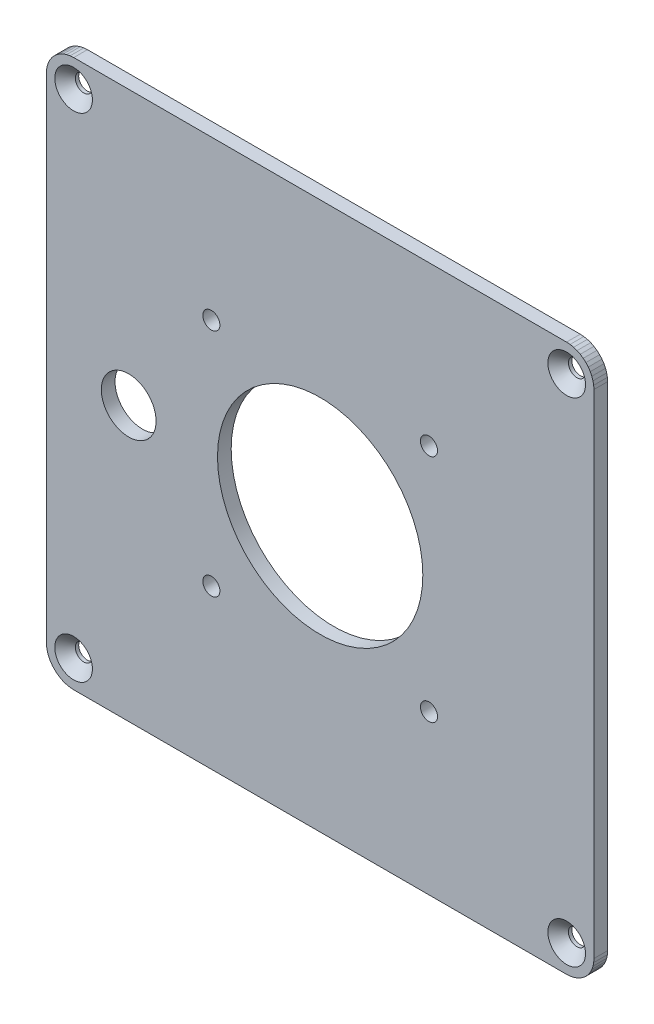
from build123d import *

# Parameters (mm, degrees)
BOSS_EXTRUDE1_DEPTH     = 2
CUT_EXTRUDE1_DEPTH      = 57.603885529
CUT_EXTRUDE1_DEPTH_BACK = 57.603885529
SKETCH2_R               = 15
SKETCH3_R               = 4
CUT_EXTRUDE2_DEPTH      = 10
SKETCH4_R               = 1.25
CUT_EXTRUDE3_DEPTH      = 10
SKETCH5_R               = 2
CUT_EXTRUDE4_DEPTH      = 10
MOVE_FACE1_BY           = 0.75
MOVE_FACE1_2_BY         = 0.75
MOVE_FACE1_3_BY         = 0.75
MOVE_FACE1_4_BY         = 0.75
CHAMFER1_SIZE           = 1.5


with BuildPart() as part:
    # Sketch1 → Boss-Extrude1 (new body)
    with BuildSketch(Plane.XY.offset(196.776792407)):
        Polygon((-39.999999106, -35.99999845), (-39.965778589, -36.522105336), (-39.863705635, -37.035275251), (-39.695519954, -37.530735135), (-39.464101195, -37.999998778), (-39.173413068, -38.43504563), (-38.828425109, -38.828425109), (-38.43504563, -39.173413068), (-37.999998778, -39.464101195), (-37.530735135, -39.695519954), (-37.035275251, -39.863705635), (-36.522105336, -39.965778589), (-35.99999845, -39.999999106), (35.99999845, -39.999999106), (36.522105336, -39.965778589), (37.035275251, -39.863705635), (37.530735135, -39.695519954), (37.999998778, -39.464101195), (38.43504563, -39.173413068), (38.828425109, -38.828425109), (39.173413068, -38.43504563), (39.464101195, -37.999998778), (39.695519954, -37.530735135), (39.863705635, -37.035275251), (39.965778589, -36.522105336), (39.999999106, -35.99999845), (39.999999106, 35.99999845), (39.965778589, 36.522105336), (39.863705635, 37.035275251), (39.695519954, 37.530735135), (39.464101195, 37.999998778), (39.173413068, 38.43504563), (38.828425109, 38.828425109), (38.43504563, 39.173413068), (37.999998778, 39.464101195), (37.530735135, 39.695519954), (37.035275251, 39.863705635), (36.522105336, 39.965778589), (35.99999845, 39.999999106), (-35.99999845, 39.999999106), (-36.522105336, 39.965778589), (-37.035275251, 39.863705635), (-37.530735135, 39.695519954), (-37.999998778, 39.464101195), (-38.43504563, 39.173413068), (-38.828425109, 38.828425109), (-39.173413068, 38.43504563), (-39.464101195, 37.999998778), (-39.695519954, 37.530735135), (-39.863705635, 37.035275251), (-39.965778589, 36.522105336), (-39.999999106, 35.99999845), align=None)
        Polygon((-37.448886782, -36.388229579), (-37.50000149, -35.99999845), (-37.448886782, -35.611771047), (-37.29903698, -35.250000656), (-37.060663104, -34.939337522), (-36.74999997, -34.700963646), (-36.388229579, -34.551113844), (-35.99999845, -34.499999136), (-35.611771047, -34.551113844), (-35.250000656, -34.700963646), (-34.939337522, -34.939337522), (-34.700963646, -35.250000656), (-34.551113844, -35.611771047), (-34.499999136, -35.99999845), (-34.551113844, -36.388229579), (-34.700963646, -36.74999997), (-34.939337522, -37.060663104), (-35.250000656, -37.29903698), (-35.611771047, -37.448886782), (-35.99999845, -37.50000149), (-36.388229579, -37.448886782), (-36.74999997, -37.29903698), (-37.060663104, -37.060663104), (-37.29903698, -36.74999997), align=None, mode=Mode.SUBTRACT)
        Polygon((-37.448886782, 35.611771047), (-37.50000149, 35.99999845), (-37.448886782, 36.388229579), (-37.29903698, 36.74999997), (-37.060663104, 37.060663104), (-36.74999997, 37.29903698), (-36.388229579, 37.448886782), (-35.99999845, 37.50000149), (-35.611771047, 37.448886782), (-35.250000656, 37.29903698), (-34.939337522, 37.060663104), (-34.700963646, 36.74999997), (-34.551113844, 36.388229579), (-34.499999136, 35.99999845), (-34.551113844, 35.611771047), (-34.700963646, 35.250000656), (-34.939337522, 34.939337522), (-35.250000656, 34.700963646), (-35.611771047, 34.551113844), (-35.99999845, 34.499999136), (-36.388229579, 34.551113844), (-36.74999997, 34.700963646), (-37.060663104, 34.939337522), (-37.29903698, 35.250000656), align=None, mode=Mode.SUBTRACT)
        Polygon((34.787815064, -36.8835181), (34.600444138, -36.539677531), (34.508455545, -36.159053445), (34.518111497, -35.767596215), (34.628756344, -35.391975194), (34.832850099, -35.057790577), (35.116482526, -34.787815064), (35.460323095, -34.600444138), (35.840947181, -34.508455545), (36.232404411, -34.518111497), (36.608025432, -34.628756344), (36.942210048, -34.832850099), (37.212185562, -35.116482526), (37.399556488, -35.460323095), (37.491541356, -35.840947181), (37.481926863, -36.232448961), (37.371270724, -36.608066656), (37.167163198, -36.942245137), (36.88352638, -37.212212123), (36.539680178, -37.399572712), (36.159053327, -37.491546138), (35.99999845, -37.48762235), (35.767596215, -37.481889129), (35.391975194, -37.371244282), (35.057790577, -37.167146802), align=None, mode=Mode.SUBTRACT)
        Polygon((34.551113844, 35.611771047), (34.499999136, 35.99999845), (34.551113844, 36.388229579), (34.700963646, 36.74999997), (34.939337522, 37.060663104), (35.250000656, 37.29903698), (35.611771047, 37.448886782), (35.99999845, 37.50000149), (36.388229579, 37.448886782), (36.74999997, 37.29903698), (37.060663104, 37.060663104), (37.29903698, 36.74999997), (37.448886782, 36.388229579), (37.50000149, 35.99999845), (37.448886782, 35.611771047), (37.29903698, 35.250000656), (37.060663104, 34.939337522), (36.74999997, 34.700963646), (36.388229579, 34.551113844), (35.99999845, 34.499999136), (35.611771047, 34.551113844), (35.250000656, 34.700963646), (34.939337522, 34.939337522), (34.700963646, 35.250000656), align=None, mode=Mode.SUBTRACT)
    extrude(amount=-BOSS_EXTRUDE1_DEPTH)

    # Sketch2 → Cut-Extrude1 (cut, two sides: drawn at the far end of the back side and taken through both)
    with BuildSketch(Plane.XY.offset(196.776792407).offset(-CUT_EXTRUDE1_DEPTH_BACK)):
        Circle(SKETCH2_R)
    extrude(amount=CUT_EXTRUDE1_DEPTH + CUT_EXTRUDE1_DEPTH_BACK, mode=Mode.SUBTRACT)

    # Sketch3 → Cut-Extrude2 (cut)
    with BuildSketch(Plane.XY.offset(196.776792407)):
        with Locations((-27.97257793, 0)):
            Circle(SKETCH3_R)
    extrude(amount=-CUT_EXTRUDE2_DEPTH, mode=Mode.SUBTRACT)

    # Sketch4 → Cut-Extrude3 (cut)
    with BuildSketch(Plane.XY.offset(196.776792407)):
        with Locations((15.898051321, 16.822185345)):
            Circle(SKETCH4_R)
        with Locations((-15.898051321, 16.822185345)):
            Circle(SKETCH4_R)
        with Locations((-15.898051321, -16.822185345)):
            Circle(SKETCH4_R)
        with Locations((15.898051321, -16.822185345)):
            Circle(SKETCH4_R)
    extrude(amount=-CUT_EXTRUDE3_DEPTH, mode=Mode.SUBTRACT)

    # Sketch5 → Cut-Extrude4 (cut)
    with BuildSketch(Plane.XY.offset(196.776792407)):
        with Locations((36.024774728, -36.000611748)):
            Circle(SKETCH5_R)
        with Locations((-36.024774728, -36.000611748)):
            Circle(SKETCH5_R)
        with Locations((-36.024774728, 36.000611748)):
            Circle(SKETCH5_R)
        with Locations((36.024774728, 36.000611748)):
            Circle(SKETCH5_R)
    extrude(amount=-CUT_EXTRUDE4_DEPTH, mode=Mode.SUBTRACT)

    # Move Face1: a curved face moved outward by 0.75
    add(Solid.thicken(part.faces().sort_by_distance((34.024774728, 36.000611748, 195.776792407))[0], MOVE_FACE1_BY))

    # Move Face1 2: a curved face moved outward by 0.75
    add(Solid.thicken(part.faces().sort_by_distance((-38.024774728, 36.000611748, 195.776792407))[0], MOVE_FACE1_2_BY))

    # Move Face1 3: a curved face moved outward by 0.75
    add(Solid.thicken(part.faces().sort_by_distance((-38.024774728, -36.000611748, 195.776792407))[0], MOVE_FACE1_3_BY))

    # Move Face1 4: a curved face moved outward by 0.75
    add(Solid.thicken(part.faces().sort_by_distance((34.024774728, -36.000611748, 195.776792407))[0], MOVE_FACE1_4_BY))

    # Chamfer1
    chamfer1_edges = [part.edges().sort_by_distance(p)[0] for p in [
        (34.774774728, 36.000611748, 196.776792407),
        (-37.274774728, 36.000611748, 196.776792407),
        (-37.274774728, -36.000611748, 196.776792407),
        (34.774774728, -36.000611748, 196.776792407),
    ]]
    chamfer(chamfer1_edges, length=CHAMFER1_SIZE)


solid = part.part
